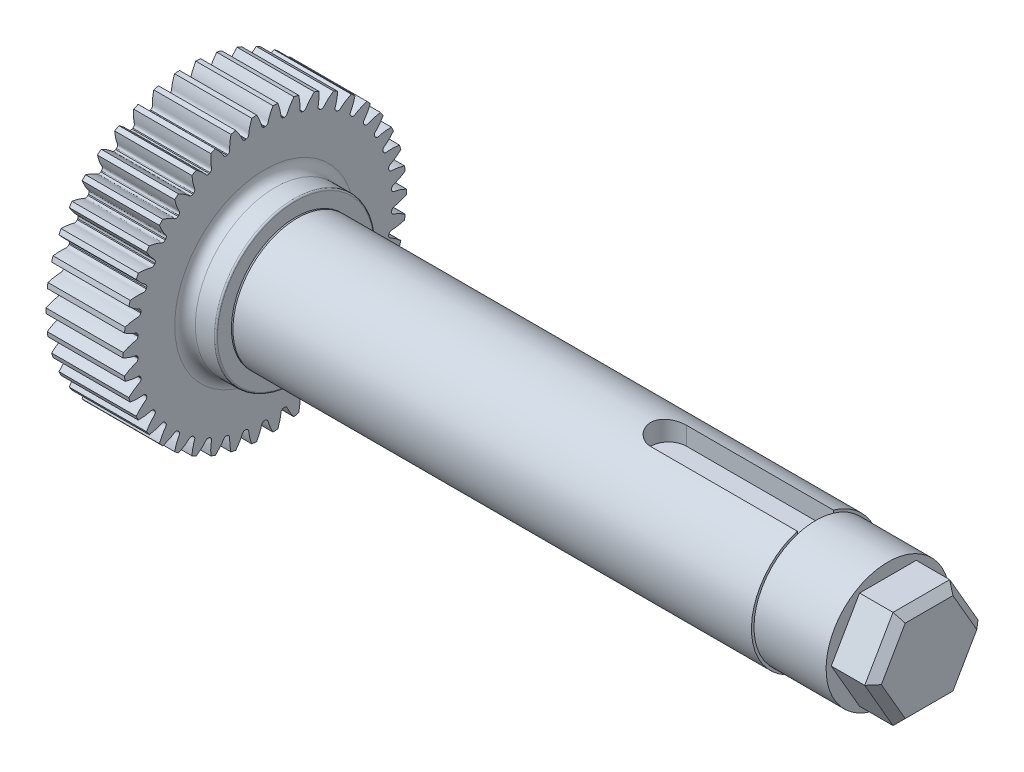
from build123d import *

# Parameters (mm, degrees)
SKETCH_1_R               = 27.5
EXTRUDE_1_DEPTH          = 15
CUT_EXTRUDE_1_DEPTH      = 15
PATTERN_CIRCULAR_1_COUNT = 42
SKETCH_3_R               = 15.5
EXTRUDE_2_DEPTH          = 6
FILLET_1_R               = 2
FILLET_2_R               = 0.3
SKETCH_4_R               = 12.25
EXTRUDE_3_DEPTH          = 0.3
SKETCH_5_R               = 12.5
EXTRUDE_4_DEPTH          = 100.7
CHAMFER_1_SIZE           = 0.25
SKETCH_6_R               = 12
EXTRUDE_5_DEPTH          = 14
EXTRUDE_6_DEPTH          = 8
CHAMFER_2_SIZE           = 1.5
CUT_EXTRUDE_2_DEPTH      = 4


with BuildPart() as part:
    # 草图1 → 凸台-拉伸1 (new body)
    with BuildSketch(Plane(origin=(0, 0, 0), x_dir=(0, 0, -1), z_dir=(1, 0, 0))):
        Circle(SKETCH_1_R)
    extrude(amount=EXTRUDE_1_DEPTH)

    # 草图2 → 切除-拉伸1 (cut)
    with BuildSketch(Plane(origin=(15, 0, 0), x_dir=(0, 0, -1), z_dir=(1, 0, 0))):
        with BuildLine():
            ThreePointArc((0.089540116, 24.687337621), (0, 24.6875), (-0.089540116, 24.687337621))
            add(Edge.make_bspline(
                [(-0.089540116, 24.687337621), (-0.562806922, 24.755684629), (-0.610811095, 25.100911679), (-0.715440192, 25.47279023), (-0.753487687, 25.599847009), (-0.797201462, 25.73545142), (-0.846795006, 25.879502778), (-0.902664725, 26.031792952), (-0.965146117, 26.192131756), (-1.034585693, 26.360309942), (-1.11131942, 26.536110281), (-1.195678673, 26.719304505), (-1.287988138, 26.909654396), (-1.38856607, 27.106911676), (-1.497723868, 27.310818254), (-1.615765858, 27.521106377), (-1.742989012, 27.73749882), (-1.879682704, 27.95970907), (-2.02612845, 28.187441523), (-2.182599664, 28.420391684), (-2.349361418, 28.658246375), (-2.5266702, 28.900683946), (-2.714773686, 29.147374497), (-2.913910513, 29.397980101), (-3.124310058, 29.652155038), (-3.346192214, 29.909546026), (-3.579767214, 30.169792468), (-3.825235318, 30.4325267), (-4.173223634, 30.790372718), (-4.445836106, 31.054176093), (-4.633336448, 31.228676668)],
                knots=[0, 0, 0, 0, 0.112031818, 0.127240278, 0.143671307, 0.161324905, 0.180201073, 0.200299811, 0.221621119, 0.244164996, 0.267931442, 0.292920459, 0.319132045, 0.3465662, 0.375222926, 0.40510222, 0.436204085, 0.468528519, 0.502075523, 0.536845096, 0.572837239, 0.610051952, 0.648489234, 0.688149086, 0.729031508, 0.771136499, 0.81446406, 0.859014191, 0.904786891, 1, 1, 1, 1], degree=3))
            ThreePointArc((-4.633336448, 31.228676668), (0, 31.570525068), (4.633336448, 31.228676668))
            add(Edge.make_bspline(
                [(0.089540116, 24.687337621), (0.562806922, 24.755684629), (0.610811095, 25.100911679), (0.715440192, 25.47279023), (0.753487687, 25.599847009), (0.797201462, 25.73545142), (0.846795006, 25.879502778), (0.902664725, 26.031792952), (0.965146117, 26.192131756), (1.034585693, 26.360309942), (1.11131942, 26.536110281), (1.195678673, 26.719304505), (1.287988138, 26.909654396), (1.38856607, 27.106911676), (1.497723868, 27.310818254), (1.615765858, 27.521106377), (1.742989012, 27.73749882), (1.879682704, 27.95970907), (2.02612845, 28.187441523), (2.182599664, 28.420391684), (2.349361418, 28.658246375), (2.5266702, 28.900683946), (2.714773686, 29.147374497), (2.913910513, 29.397980101), (3.124310058, 29.652155038), (3.346192214, 29.909546026), (3.579767214, 30.169792468), (3.825235318, 30.4325267), (4.173223634, 30.790372718), (4.445836106, 31.054176093), (4.633336448, 31.228676668)],
                knots=[0, 0, 0, 0, 0.112031818, 0.127240278, 0.143671307, 0.161324905, 0.180201073, 0.200299811, 0.221621119, 0.244164996, 0.267931442, 0.292920459, 0.319132045, 0.3465662, 0.375222926, 0.40510222, 0.436204085, 0.468528519, 0.502075523, 0.536845096, 0.572837239, 0.610051952, 0.648489234, 0.688149086, 0.729031508, 0.771136499, 0.81446406, 0.859014191, 0.904786891, 1, 1, 1, 1], degree=3))
        make_face()
    cut_extrude_1 = extrude(amount=-CUT_EXTRUDE_1_DEPTH, mode=Mode.SUBTRACT)

    # 阵列(圆周)1: 切除-拉伸1 ×42 about axis
    pattern_circular_1_axis = Axis((88.99, 0, 0), (-1, 0, 0))
    for i in range(1, PATTERN_CIRCULAR_1_COUNT):
        add(cut_extrude_1.rotate(pattern_circular_1_axis, i * 360 / PATTERN_CIRCULAR_1_COUNT), mode=Mode.SUBTRACT)

    # 草图3 → 凸台-拉伸2 (add)
    with BuildSketch(Plane(origin=(15, 0, 0), x_dir=(0, 0, -1), z_dir=(1, 0, 0))):
        Circle(SKETCH_3_R)
    extrude(amount=EXTRUDE_2_DEPTH)

    # 圆角1
    fillet_1_edges = [part.edges().sort_by_distance(p)[0] for p in [
        (15, 0, 15.5),
    ]]
    fillet(fillet_1_edges, radius=FILLET_1_R)

    # 圆角2
    fillet_2_edges = [part.edges().sort_by_distance(p)[0] for p in [
        (21, 0, 15.5),
    ]]
    fillet(fillet_2_edges, radius=FILLET_2_R)

    # 草图4 → 凸台-拉伸3 (add)
    with BuildSketch(Plane(origin=(21, 0, 0), x_dir=(0, 0, -1), z_dir=(1, 0, 0))):
        Circle(SKETCH_4_R)
    extrude(amount=EXTRUDE_3_DEPTH)

    # 草图5 → 凸台-拉伸4 (add)
    with BuildSketch(Plane(origin=(21.3, 0, 0), x_dir=(0, 0, -1), z_dir=(1, 0, 0))):
        Circle(SKETCH_5_R)
    extrude(amount=EXTRUDE_4_DEPTH)

    # 倒角1
    chamfer_1_edges = [part.edges().sort_by_distance(p)[0] for p in [
        (21, 0, 12.25),
    ]]
    chamfer(chamfer_1_edges, length=CHAMFER_1_SIZE)

    # 草图6 → 凸台-拉伸5 (add)
    with BuildSketch(Plane(origin=(122, 0, 0), x_dir=(0, 0, -1), z_dir=(1, 0, 0))):
        Circle(SKETCH_6_R)
    extrude(amount=EXTRUDE_5_DEPTH)

    # 草图9 → 凸台-拉伸6 (add)
    with BuildSketch(Plane(origin=(136, 0, 0), x_dir=(0, 0, -1), z_dir=(1, 0, 0))):
        Polygon((11, 0), (5.5, 9.526279442), (-5.5, 9.526279442), (-11, 0), (-5.5, -9.526279442), (5.5, -9.526279442), align=None)
    extrude(amount=EXTRUDE_6_DEPTH)

    # 倒角2
    chamfer_2_edges = [part.edges().sort_by_distance(p)[0] for p in [
        (144, -4.763139721, -8.25),
        (144, 4.763139721, -8.25),
        (144, 9.526279442, 0),
        (144, 4.763139721, 8.25),
        (144, -4.763139721, 8.25),
        (144, -9.526279442, 0),
    ]]
    chamfer(chamfer_2_edges, length=CHAMFER_2_SIZE)

    # 草图11 → 切除-拉伸2 (cut)
    with BuildSketch(Plane(origin=(0, 12.5, 0), x_dir=(1, 0, 0), z_dir=(0, 1, 0))):
        with BuildLine():
            Line((122, -3.589540116), (122, 3.410459884))
            Line((122, 3.410459884), (93.5, 3.410459884))
            ThreePointArc((93.5, 3.410459884), (90, -0.089540116), (93.5, -3.589540116))
            Line((93.5, -3.589540116), (122, -3.589540116))
        make_face()
    extrude(amount=-CUT_EXTRUDE_2_DEPTH, mode=Mode.SUBTRACT)


solid = part.part
